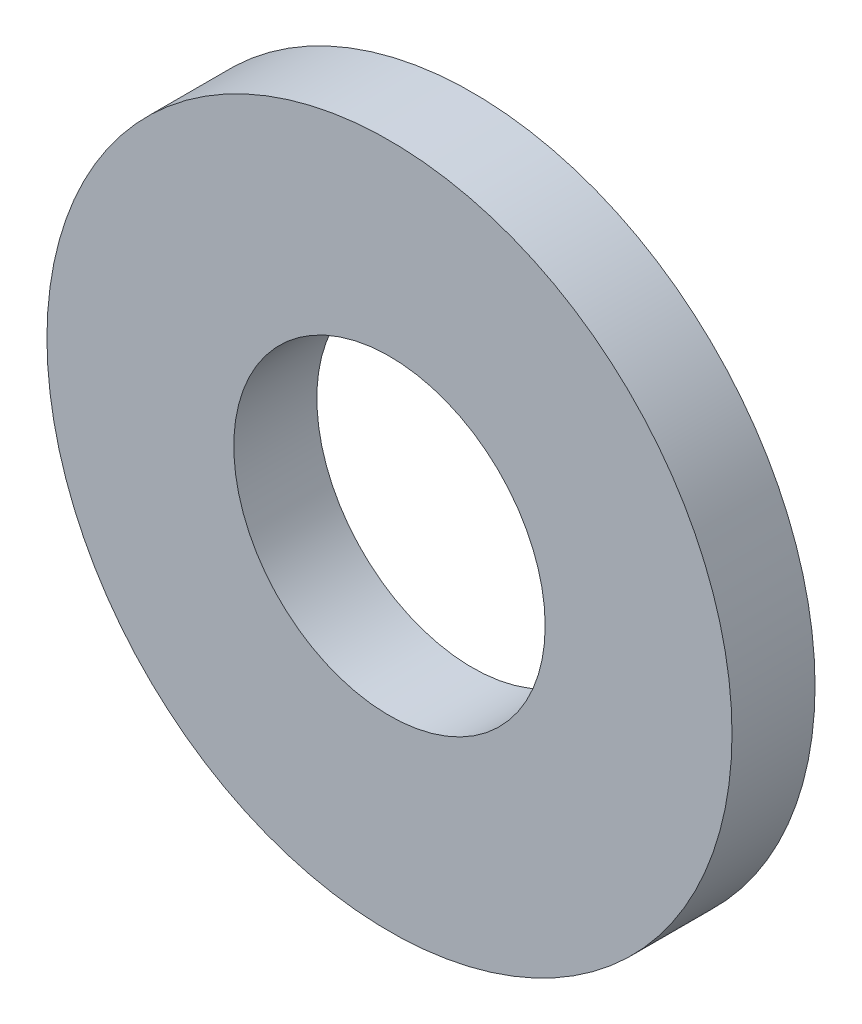
from build123d import *

# Parameters (mm, degrees)
SKETCH1_R           = 82.5
SKETCH1_R_2         = 37.5
BOSS_EXTRUDE1_DEPTH = 20


with BuildPart() as part:
    # Sketch1 → Boss-Extrude1 (new body)
    with BuildSketch(Plane.XY):
        Circle(SKETCH1_R)
        Circle(SKETCH1_R_2, mode=Mode.SUBTRACT)
    extrude(amount=BOSS_EXTRUDE1_DEPTH)


solid = part.part
